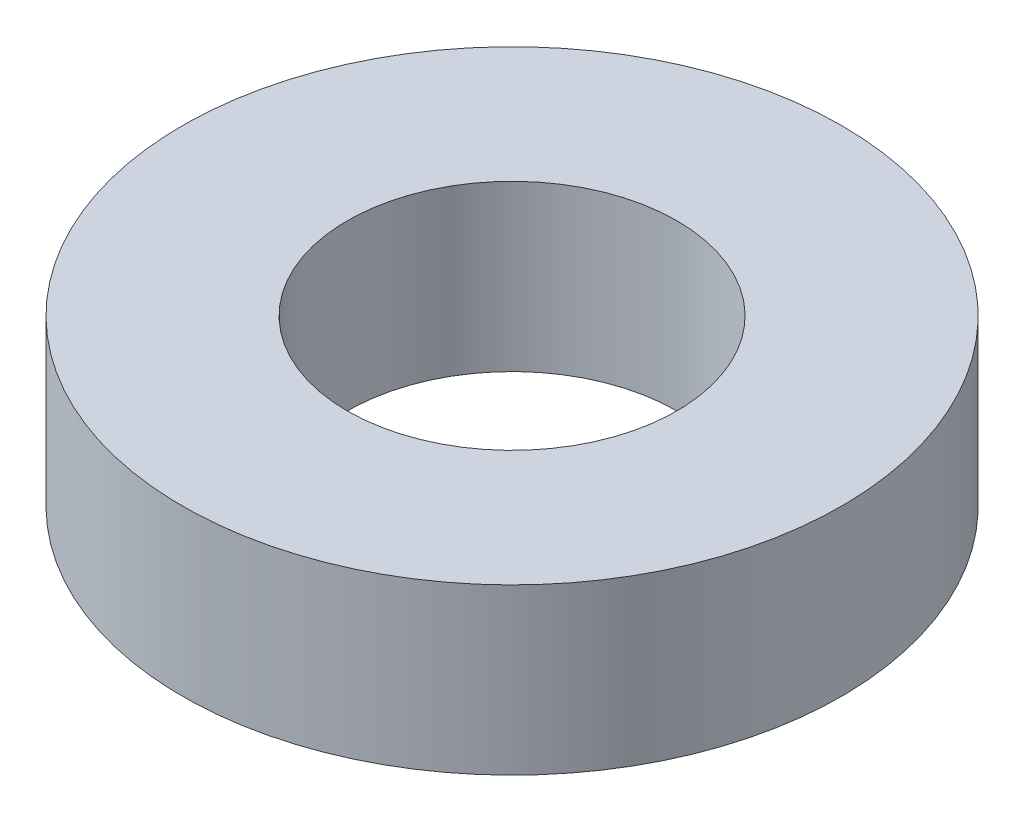
SolidWorks part; units mm, degrees
ref_plane "前视基准面" through (0, 0, 0) normal (0, 0, 1) x (1, 0, 0)
ref_plane "上视基准面" through (0, 0, 0) normal (0, 1, 0) x (1, 0, 0)
ref_plane "右视基准面" through (0, 0, 0) normal (1, 0, 0) x (0, 0, -1)
sketch "草图1" plane through (0, 0, 0) normal (0, 0, 1) x (1, 0, 0)
  line L0 (0, 0) -> (0, 12045.1507) construction
  line L1 (4, 1.0997) -> (8, 1.0997)
  line L2 (8, 1.0997) -> (8, -2.9003)
  line L3 (8, -2.9003) -> (4, -2.9003)
  line L4 (4, -2.9003) -> (4, 1.0997)
  dimension "D1" = 4
  dimension "D2" = 4
  dimension "D3" = 4
revolve "旋转1" add sketch "草图1" angle 360 about L0
